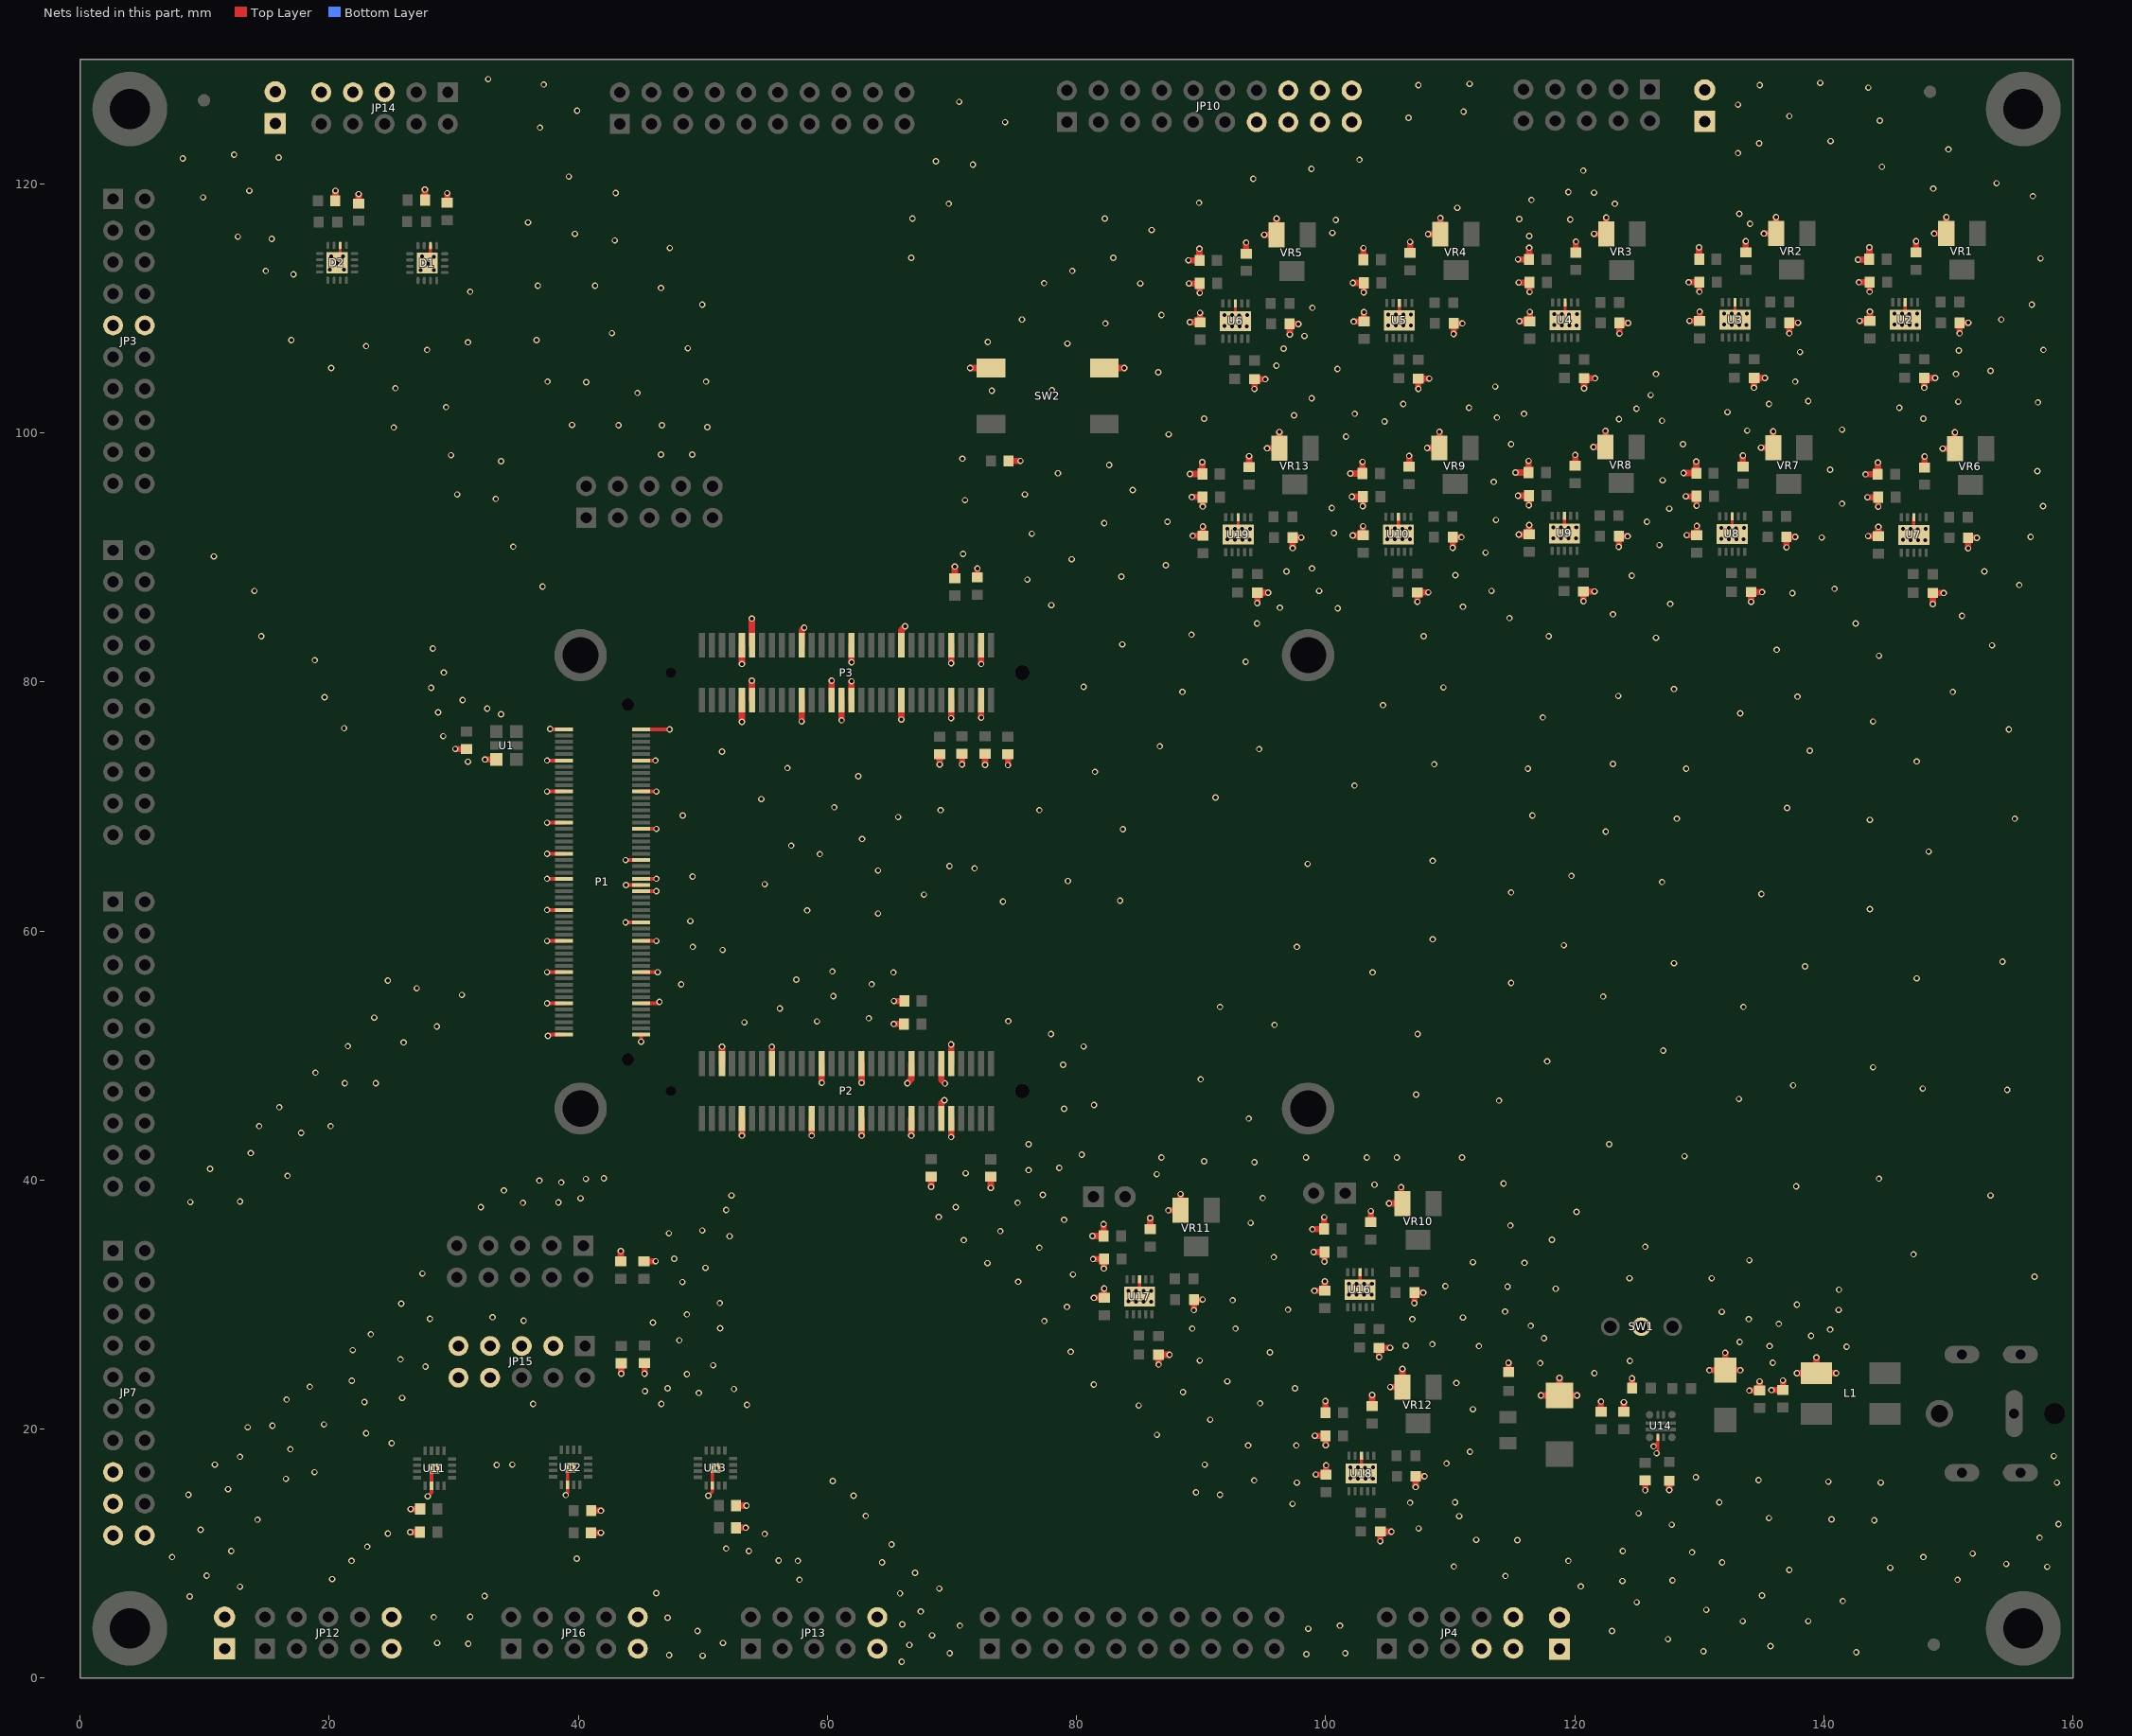
[diagram p0: the nets of this part, all layers, seen from the top]
# Altium PCB MISC82195.PcbDoc (part 4 of 8)
Units mm, origin at the board's own origin, x right, y up, seen from the top; angles counter-clockwise.
Board outline 160 x 130 mm, 4 copper layers (Top Layer, GND, POWER, Bottom Layer); 214 components, 251 nets, 1068 pads, 1218 vias.

## Via types
v1: diameter 0.508, hole 0.305, Top Layer to Bottom Layer, 1218 vias

## Nets (pads, with @x,y where several pads share a name; then routed paths per layer and width w, separated by ;. In a path a pad name is that pad's centre, name@x,y a point inside that pad or via, vN(x,y) a via of type N, cw(c..) or ccw(c..) an arc to the next point about the centre after c; other vN are vias at no path point) (continued)
GND: C1.2 C2.1 C3.1 C4.1 C5.1 C6.1 C7.1 C8.2 C9.1 C10.1 C11.1 C12.2 C13.1 C14.1 C15.1 C16.1 C17.1 C18.1 C19.1 C20.1 C21.1 C22.1 C23.1 C24.1 C25.1 C26.1 C27.1 C28.1 C29.1 C30.1 C31.1 C32.1 C33.1 C34.1 C35.1 C36.1 C37.1 C38.1 C39.1 C40.1 C41.1 C42.1 C43.1 C44.1 C45.1 C46.1 C47.1 C48.1 C49.1 C50.1 C51.1 C52.1 C53.1 C54.1 C55.1 C56.1 C57.1 C58.2 C59.1 C60.2 C61.1 C62.1 C63.1 C64.1 C65.1 C66.1 C67.1 C68.1 C69.1 C70.1 C71.1 C72.1 C73.1 C74.1 C75.1 C76.1 C77.1 C78.1 C79.1 C80.1 C81.1 C82.1 C83.1 D1.14 D1.17 D2.14 D2.17 D3.2 D4.1 JP3.9 JP3.10 JP4.7 JP4.9 JP4.10 JP7.15 JP7.17 JP7.19 JP7.20 JP10.13 JP10.15 JP10.16 JP10.17 JP10.18 JP10.19 JP10.20 JP12.9 JP12.10 JP13.9 JP13.10 JP14.5 JP14.7 JP14.9 JP15.3 JP15.5 JP15.7 JP15.8 JP15.9 JP15.10 JP16.9 JP16.10 JP17.1 JP17.2 JP18.1 JP18.2 JP20.1 JP20.2 JP21.1 JP21.2 L1.3 P1.B1 P1.B2 P1.B11 P1.B12 P1.B21 P1.B22 P1.B32 P1.B33 P1.B42 P1.B43 P1.B49 P1.B50 P1.B51 P1.B53 P1.B60 P1.B63 P1.B69 P1.B70 P1.B79 P1.B80 P1.B89 P1.B90 P1.B99 P1.B100 P2.A5 P2.A10 P2.A15 P2.A24 P2.A25 P2.A33 P2.A34 P2.A43 P2.A44 P2.A49 P2.A50 P2.A51 P2.A52 P3.C9 P3.C10 P3.C11 P3.C12 P3.C21 P3.C22 P3.C28 P3.C30 P3.C31 P3.C32 P3.C41 P3.C42 P3.C51 P3.C52 P3.C57 P3.C58 R7.1 R8.1 R9.1 R10.1 R11.1 R12.1 R19.1 R20.1 R21.1 R22.1 R23.1 R24.1 R31.1 R32.1 R33.1 R34.1 R35.1 R36.1 R39.2 R40.2 R42.1 R49.1 R50.1 R51.1 R52.1 R53.1 R54.1 R57.1 R58.1 SW1.2 SW2.1 SW2.2 U1.3 U2.8 U2.11 U3.8 U3.11 U4.8 U4.11 U5.8 U5.11 U6.8 U6.11 U7.8 U7.11 U8.8 U8.11 U9.8 U9.11 U10.8 U10.11 U11.6 U11.17 U12.6 U12.17 U13.6 U13.17 U14.8 U16.8 U16.11 U17.8 U17.11 U18.8 U18.11 U19.8 U19.11 VR1.3 VR2.3 VR3.3 VR4.3 VR5.3 VR6.3 VR7.3 VR8.3 VR9.3 VR10.3 VR11.3 VR12.3 VR13.3 | length 287.4
  Top Layer w0.254: D2.17@20.891,114.465 D2.14@20.891,115.05 ; D1.17@28.13,114.312 D1.14@28.13,115.024 ; U17.11@85.057,31.387 U17.8@85.057,32.044 ; 92.753,109.771 U6.8@92.753,110.377 ; U19.11@92.982,92.616 U19.8@92.982,93.232 ; U16.11@102.761,31.986 U16.8@102.761,32.603 ; U18.11@102.862,17.188 U18.8@102.862,17.845 ; U10.11@105.834,92.601 U10.8@105.834,93.258 ; U5.11@105.91,109.812 U5.8@105.91,110.428 ; U9.11@119.169,92.667 U9.8@119.169,93.334 ; U4.11@119.22,109.812 U4.8@119.22,110.454 ; v1(126.314,18.618) 126.34,18.618 126.673,18.952 U14.8@126.673,19.339 126.673,18.165 v1(126.568,18.059) ; U8.11@132.631,92.626 U8.8@132.631,93.283 ; U3.11@132.86,109.837 U3.8@132.86,110.479 ; 146.525,109.873 U2.8@146.525,110.479 ; U7.11@147.211,92.565 U7.8@147.211,93.207
  Top Layer w0.279: v1(27.915,14.605) 28.214,14.905 U11.6@28.214,15.443 U11.17@28.214,16.505 ; v1(38.989,14.707) 39.136,14.854 U12.6@39.136,15.519 U12.17@39.136,16.657 ; v1(50.444,14.656) 50.769,14.981 U13.6@50.769,15.468 U13.17@50.769,16.556
  Top Layer w0.305: v1(37.498,54.188) P1.B90@38.866,54.188 ; v1(37.498,56.688) P1.B80@38.866,56.688 ; v1(37.498,59.188) P1.B70@38.866,59.188 ; v1(37.498,61.688) P1.B60@38.866,61.688 ; v1(37.498,64.188) P1.B50@38.866,64.188 ; v1(37.498,66.188) P1.B42@38.866,66.188 ; v1(37.498,68.688) P1.B32@38.866,68.688 ; v1(37.498,71.188) P1.B22@38.866,71.188 ; v1(37.498,73.688) P1.B12@38.866,73.688 ; v1(37.567,51.562) 37.693,51.688 P1.B100@38.866,51.688 ; v1(37.744,76.225) 37.781,76.188 P1.B2@38.866,76.188 ; v1(43.803,60.688) P1.B63@45.038,60.688 ; v1(43.803,65.688) P1.B43@45.038,65.688 ; v1(43.826,63.688) P1.B51@45.038,63.688 ; v1(45.038,51.101) P1.B99@45.038,51.688 ; P1.B89@45.038,54.188 46.391,54.188 v1(46.507,54.305) ; P1.B79@45.038,56.688 v1(46.376,56.688) ; P1.B69@45.038,59.188 v1(46.274,59.188) ; P1.B53@45.038,63.188 v1(46.274,63.188) ; P1.B49@45.038,64.188 v1(46.274,64.188) ; P1.B33@45.038,68.188 v1(46.274,68.188) ; P1.B21@45.038,71.188 v1(46.274,71.188) ; P1.B11@45.038,73.688 v1(46.2,73.688) ; P1.B1@45.038,76.188 v1(47.334,76.188)
  Top Layer w0.508: C59.1@20.503,118.628 v1(20.503,119.436) ; C60.2@22.368,118.414 v1(22.368,119.168) ; v1(26.502,11.72) C50.1@27.282,11.72 ; v1(26.553,13.574) C49.1@27.307,13.574 ; C57.1@27.691,118.679 v1(27.691,119.537) ; C58.2@29.48,118.465 v1(29.48,119.244) ; v1(30.136,74.611) C1.2@31.039,74.611 ; v1(32.515,73.764) U1.3@33.43,73.764 ; C52.1@41.019,11.674 v1(41.819,11.674) ; C51.1@41.044,13.452 v1(41.819,13.452) ; C56.1@43.418,33.481 v1(43.418,34.299) ; v1(43.443,24.444) C61.1@43.443,25.285 ; C55.1@45.272,33.481 v1(46.207,33.481) ; v1(45.323,24.444) C62.1@45.323,25.311 ; P2.A5@51.537,49.338 v1(51.537,50.707) ; C53.1@52.678,12.08 v1(53.452,12.08) ; C54.1@52.678,13.858 v1(53.503,13.858) ; v1(53.137,43.57) P2.A10@53.137,44.938 ; v1(53.137,76.785) P3.C10@53.137,78.539 ; v1(53.137,81.433) P3.C9@53.137,82.939 ; P3.C12@53.937,78.539 v1(53.937,80.099) ; P3.C11@53.937,82.939 v1(53.937,85.078) ; P2.A15@55.537,49.338 v1(55.537,50.707) ; v1(57.937,76.81) P3.C22@57.937,78.539 ; P3.C21@57.937,82.939 57.937,84.15 v1(58.141,84.353) ; v1(58.737,43.57) P2.A24@58.737,44.938 ; v1(59.537,47.803) P2.A25@59.537,49.338 ; P3.C28@60.337,78.539 v1(60.337,80.099) ; v1(61.137,76.912) P3.C30@61.137,78.539 ; P3.C32@61.937,78.539 v1(61.937,80.048) ; v1(61.937,81.573) P3.C31@61.937,82.939 ; v1(62.737,43.57) P2.A34@62.737,44.938 ; v1(62.737,47.803) P2.A33@62.737,49.338 ; v1(65.329,52.527) C6.1@66.153,52.527 ; v1(65.345,54.372) C4.1@66.168,54.372 ; v1(65.937,76.963) P3.C42@65.937,78.539 ; P3.C41@65.937,82.939 65.937,84.149 v1(66.243,84.455) ; v1(66.421,47.777) 66.737,48.094 P2.A43@66.737,49.338 ; v1(66.737,43.57) P2.A44@66.737,44.938 ; v1(68.326,39.446) C5.1@68.326,40.27 ; v1(69.012,73.355) C12.2@69.012,74.205 ; P2.A50@69.137,44.938 69.137,46.15 v1(69.393,46.406) ; P2.A49@69.137,49.338 69.137,48.058 v1(69.444,47.752) ; v1(69.937,43.448) P2.A52@69.937,44.938 ; P2.A51@69.937,49.338 v1(69.937,50.887) ; v1(69.937,77.078) P3.C52@69.937,78.539 ; v1(69.937,81.497) P3.C51@69.937,82.939 ; C11.1@70.231,88.33 v1(70.231,89.256) ; v1(70.806,73.371) C9.1@70.806,74.215 ; v1(71.461,105.196) SW2.1@73.123,105.196 ; C10.1@72.034,88.381 v1(72.034,89.103) ; v1(72.337,77.116) P3.C58@72.337,78.539 ; v1(72.337,81.434) P3.C57@72.337,82.939 ; v1(72.66,73.339) C2.1@72.66,74.215 ; v1(73.117,39.361) C7.1@73.117,40.255 ; v1(74.489,73.314) C3.1@74.489,74.189 ; C8.2@74.538,97.739 v1(75.489,97.739) ; v1(81.28,35.509) C72.1@82.274,35.509 ; v1(81.331,33.655) C73.1@82.198,33.655 v1(82.198,32.896) ; v1(81.393,30.545) C71.1@82.22,30.545 v1(82.22,31.293) ; C72.1@82.172,35.509 v1(82.172,36.452) ; SW2.2@82.223,105.196 v1(83.835,105.196) ; C78.1@85.92,36.057 v1(85.92,36.939) ; v1(86.581,25.179) R53.1@86.581,25.967 v1(87.461,25.967) ; v1(87.374,37.569) VR11.3@88.353,37.569 v1(88.353,38.874) ; v1(88.976,113.843) C29.1@89.869,113.843 v1(89.869,114.786) ; v1(89.027,111.989) C30.1@89.894,111.989 v1(89.894,111.23) ; v1(89.089,108.879) C28.1@89.916,108.879 v1(89.916,109.626) ; v1(89.103,96.698) C81.1@90.097,96.698 v1(90.097,97.641) ; v1(89.256,94.844) C82.1@90.123,94.844 v1(90.123,94.085) ; v1(89.318,91.734) C80.1@90.145,91.734 v1(90.145,92.481) ; v1(89.417,29.549) R50.1@89.417,30.404 v1(90.119,30.404) ; C35.1@93.617,114.39 v1(93.617,115.273) ; C83.1@93.845,97.245 v1(93.845,98.128) ; v1(94.277,103.513) R23.1@94.277,104.301 v1(95.157,104.301) ; v1(94.506,86.327) R58.1@94.506,87.156 v1(95.386,87.156) ; v1(95.07,115.902) VR5.3@96.05,115.902 v1(96.05,117.208) ; v1(95.299,98.757) VR13.3@96.278,98.757 v1(96.278,100.063) ; v1(97.113,107.883) R20.1@97.113,108.737 v1(97.815,108.737) ; v1(97.342,90.738) R57.1@97.342,91.592 v1(98.044,91.592) ; v1(98.933,36.043) C69.1@99.927,36.043 ; v1(99.035,34.214) C70.1@99.902,34.214 v1(99.902,33.455) ; v1(99.097,31.104) C68.1@99.924,31.104 v1(99.924,31.852) ; v1(99.136,19.456) C76.1@100.003,19.456 v1(100.003,18.698) ; v1(99.198,16.346) C74.1@100.025,16.346 v1(100.025,17.094) ; C69.1@99.876,36.068 v1(99.876,37.011) ; C75.1@99.978,21.311 v1(99.978,22.254) ; v1(101.981,96.723) C44.1@102.975,96.723 ; v1(102.108,94.869) C45.1@102.975,94.869 v1(102.975,94.11) ; v1(102.17,91.759) C43.1@102.997,91.759 v1(102.997,92.507) ; v1(102.184,112.039) C27.1@103.051,112.039 v1(103.051,111.281) ; v1(102.246,108.929) C25.1@103.073,108.929 v1(103.073,109.677) ; C44.1@102.95,96.723 v1(102.95,97.666) ; C26.1@103.026,113.894 v1(103.026,114.837) ; C77.1@103.624,36.616 v1(103.624,37.498) ; C79.1@103.726,21.858 v1(103.726,22.741) ; v1(104.285,25.773) R52.1@104.285,26.526 v1(105.165,26.526) ; v1(104.386,10.99) R54.1@104.386,11.769 v1(105.266,11.769) ; v1(105.078,38.128) 106.057,38.128 v1(106.057,39.433) ; v1(105.179,23.37) VR12.3@106.159,23.37 ; VR12.3@106.159,23.523 v1(106.159,24.828) ; C48.1@106.698,97.271 v1(106.698,98.153) ; C34.1@106.774,114.441 v1(106.774,115.324) ; v1(107.121,30.108) R49.1@107.121,30.963 v1(107.823,30.963) ; v1(107.222,15.351) R51.1@107.222,16.205 v1(107.925,16.205) ; v1(107.358,86.419) R36.1@107.358,87.181 v1(108.238,87.181) ; v1(107.434,103.523) R22.1@107.434,104.352 v1(108.314,104.352) ; v1(108.151,98.783) VR9.3@109.131,98.783 v1(109.131,100.088) ; v1(108.227,115.953) VR4.3@109.207,115.953 v1(109.207,117.259) ; v1(110.194,90.763) R33.1@110.194,91.618 v1(110.896,91.618) ; v1(110.27,107.934) R19.1@110.27,108.788 v1(110.973,108.788) ; R42.1@114.681,24.579 v1(114.681,25.324) ; v1(115.24,96.799) C41.1@116.234,96.799 ; v1(115.443,94.945) C42.1@116.31,94.945 v1(116.31,94.187) ; v1(115.443,113.919) C20.1@116.437,113.919 ; v1(115.494,112.065) C21.1@116.361,112.065 v1(116.361,111.306) ; v1(115.505,91.835) C40.1@116.332,91.835 v1(116.332,92.583) ; v1(115.556,108.955) C19.1@116.383,108.955 v1(116.383,109.703) ; C41.1@116.285,96.799 v1(116.285,97.743) ; C20.1@116.335,113.919 v1(116.335,114.862) ; v1(117.273,22.706) D3.2@118.77,22.706 ; v1(118.77,24.105) D3.2@118.77,22.706 ; C47.1@120.033,97.347 v1(120.033,98.23) ; C24.1@120.083,114.467 v1(120.083,115.349) ; v1(120.191,22.706) D3.2@118.77,22.706 ; v1(120.693,86.469) R35.1@120.693,87.258 v1(121.573,87.258) ; v1(120.744,103.564) R12.1@120.744,104.377 v1(121.624,104.377) ; v1(121.486,98.859) VR8.3@122.466,98.859 v1(122.466,100.164) ; v1(121.537,115.979) VR3.3@122.516,115.979 v1(122.516,117.284) ; C64.1@122.098,21.401 v1(122.098,22.225) ; v1(123.529,90.839) R32.1@123.529,91.694 v1(124.231,91.694) ; v1(123.58,107.959) R9.1@123.58,108.814 v1(124.282,108.814) ; C63.1@123.936,21.391 v1(123.936,22.158) ; R39.2@124.596,23.292 v1(124.596,24.071) ; v1(125.654,15.088) C67.1@125.654,15.886 ; v1(127.584,15.113) R40.2@127.584,15.858 ; v1(128.727,96.774) C38.1@129.721,96.774 ; v1(128.905,94.894) C39.1@129.772,94.894 v1(129.772,94.136) ; v1(128.967,91.784) C37.1@129.794,91.784 v1(129.794,92.532) ; v1(129.134,112.09) C18.1@130.001,112.09 v1(130.001,111.332) ; v1(129.196,108.98) C16.1@130.023,108.98 v1(130.023,109.728) ; C38.1@129.747,96.749 v1(129.747,97.692) ; C17.1@129.975,113.944 v1(129.975,114.888) ; v1(130.791,24.733) D4.1@132.08,24.733 ; v1(132.08,26.137) D4.1@132.08,24.733 ; v1(133.293,24.733) D4.1@132.08,24.733 ; C46.1@133.495,97.296 v1(133.495,98.179) ; C23.1@133.723,114.492 v1(133.723,115.375) ; v1(134.006,23.093) C66.1@134.832,23.093 v1(134.832,23.834) ; v1(134.155,86.419) R34.1@134.155,87.207 v1(135.035,87.207) ; v1(134.384,103.614) R11.1@134.384,104.403 v1(135.264,104.403) ; v1(134.948,98.808) VR7.3@135.928,98.808 v1(135.928,100.114) ; v1(135.177,116.004) VR2.3@136.156,116.004 v1(136.156,117.309) ; v1(135.777,23.128) C65.1@136.703,23.128 v1(136.703,23.901) ; v1(136.991,90.789) R31.1@136.991,91.643 v1(137.693,91.643) ; v1(137.22,107.984) R8.1@137.22,108.839 v1(137.922,108.839) ; v1(137.82,24.485) L1.3@139.388,24.485 ; v1(139.388,25.749) L1.3@139.388,24.485 ; v1(140.969,24.485) L1.3@139.388,24.485 ; v1(142.723,113.894) C14.1@143.717,113.894 ; v1(142.799,112.09) C15.1@143.666,112.09 v1(143.666,111.332) ; v1(142.861,108.98) C13.1@143.688,108.98 v1(143.688,109.728) ; v1(143.332,96.672) C32.1@144.326,96.672 v1(144.326,97.616) ; v1(143.485,94.818) C33.1@144.352,94.818 v1(144.352,94.06) ; v1(143.547,91.708) C31.1@144.374,91.708 v1(144.374,92.456) ; C14.1@143.64,113.944 v1(143.64,114.888) ; C22.1@147.388,114.492 v1(147.388,115.375) ; v1(148.049,103.614) R10.1@148.049,104.403 v1(148.929,104.403) ; C36.1@148.074,97.22 v1(148.074,98.103) ; v1(148.735,86.241) R24.1@148.735,87.131 v1(149.615,87.131) ; v1(148.842,116.004) VR1.3@149.821,116.004 v1(149.821,117.309) ; v1(149.528,98.732) VR6.3@150.507,98.732 v1(150.507,100.037) ; v1(150.885,107.984) R7.1@150.885,108.839 v1(151.587,108.839) ; v1(151.571,90.712) R21.1@151.571,91.567 v1(152.273,91.567)
  Bottom Layer w0.305: v1@37.719,76.2 v1(37.744,76.225)
  other v1: 65.964,1.321 49.987,1.803 47.295,1.854 98.45,1.93 69.825,2.007 101.575,2.007 142.596,2.083 130.327,2.159 135.712,2.565 66.573,2.667 31.166,2.769 28.677,2.819 51.613,2.819 127.483,3.124 68.402,3.429 49.581,3.785 122.987,3.785 98.603,3.962 70.637,4.216 101.143,4.216 66.015,4.318 133.477,4.572 138.735,4.572 47.168,4.851 28.397,4.902 31.318,4.928 67.488,5.359 130.556,5.486 124.968,6.096 141.503,6.198 8.814,6.553 32.487,6.604 135.026,6.629 65.837,6.807 46.253,6.833 68.986,7.188 12.852,7.341 120.472,7.366 123.825,7.798 127.838,7.849 57.76,7.899 150.724,7.899 20.244,7.95 114.427,8.204 10.16,8.23 67.031,8.458 137.211,8.687 145.313,8.865 157.912,8.941 110.287,8.966 154.635,9.169 64.389,9.296 131.826,9.296 21.793,9.423 57.633,9.423 119.482,9.423 56.083,9.449 39.878,9.601 7.391,9.728 147.98,9.728 151.943,10.008 129.413,10.109 12.141,10.211 53.696,10.211 123.85,10.211 51.867,10.414 23.063,10.566 65.151,10.744 115.392,11.074 112.09,11.1 157.302,11.278 54.966,11.582 24.714,11.608 9.677,11.913 107.467,12.014 127.787,12.319 158.826,12.37 144.043,12.675 14.249,12.725 140.614,12.751 135.585,12.852 110.719,13.005 63.068,13.03 125.12,13.233 97.333,13.995 106.782,14.097 110.388,14.122 131.597,14.122 62.103,14.656 8.712,14.732 91.516,14.732 89.586,14.91 11.887,15.164 97.688,15.697 144.551,15.697 158.699,15.697 140.36,15.773 60.427,15.824 94.259,15.875 134.747,15.9 16.535,16.002 102.591,16.027 103.2,16.027 103.784,16.027 101.981,16.053 129.718,16.129 18.821,16.535 28.473,16.84 51.029,16.84 103.175,16.891 39.395,16.916 101.981,16.916 102.591,16.916 103.81,16.916 33.452,17.12 10.82,17.145 34.696,17.145 90.297,17.145 109.703,17.247 12.852,17.78 158.445,17.831 111.582,18.186 16.891,18.39 93.777,18.694 97.638,18.694 25.019,18.872 86.462,19.533 22.962,19.66 13.462,20.142 15.443,20.269 19.583,20.371 90.729,20.752 111.811,21.59 84.988,21.895 53.543,21.946 36.373,22.022 46.66,22.022 94.742,22.073 22.835,22.174 16.586,22.377 25.857,22.504 49.682,22.911 88.544,22.962 45.364,23.038 52.502,23.216 47.168,23.266 97.536,23.266 18.44,23.393 81.382,23.571 110.49,23.698 92.1,23.825 21.819,23.876 48.717,24.409 121.564,24.486 27.737,25.019 50.825,25.121 117.221,25.298 135.89,25.324 124.409,25.476 89.891,25.502 25.73,25.603 95.529,26.162 79.527,26.213 21.895,26.34 141.808,26.619 112.293,26.67 135.636,26.67 106.426,26.695 108.56,26.822 133.223,27 48.108,27.127 117.526,27.305 138.963,27.483 23.343,27.61 140.487,27.991 89.281,28.067 92.761,28.067 51.384,28.092 116.459,28.296 136.373,28.448 45.999,28.55 77.419,28.677 35.611,28.702 106.959,28.829 133.96,28.829 28.092,28.854 111.023,28.956 33.122,28.981 48.717,29.21 131.801,29.413 114.402,29.439 141.173,29.566 96.977,29.591 79.223,29.82 137.82,29.997 25.781,30.074 51.359,30.124 84.785,30.226 85.395,30.226 85.979,30.226 84.176,30.251 92.532,30.353 102.489,30.785 103.099,30.785 103.683,30.785 101.879,30.81 85.369,31.09 84.176,31.115 84.785,31.115 86.004,31.115 141.199,31.191 118.466,31.267 114.605,31.445 109.601,31.471 103.073,31.648 101.879,31.674 102.489,31.674 103.708,31.674 48.362,31.801 75.311,31.826 124.384,32.106 130.988,32.106 156.896,32.233 79.705,32.41 27.483,32.487 50.216,32.944 72.847,33.325 115.951,33.35 111.811,33.401 134.01,33.553 47.701,33.68 95.834,33.807 147.193,34.036 77.013,34.569 125.654,34.646 70.942,35.179 118.161,35.204 52.146,35.484 47.269,35.712 73.889,35.89 49.962,35.941 114.833,36.347 93.98,36.551 78.994,36.805 68.936,37.033 120.142,37.44 51.867,37.592 32.182,37.821 70.307,37.821 35.56,38.176 75.26,38.176 38.405,38.202 8.865,38.227 12.852,38.278 40.183,38.532 94.945,38.557 52.299,38.76 153.365,38.76 77.292,38.811 34.036,39.167 137.77,39.497 103.911,39.624 114.275,39.726 38.633,39.802 36.881,39.954 40.615,40.081 144.424,40.107 42.062,40.132 16.662,40.335 86.436,40.462 71.095,40.538 76.149,40.792 10.439,40.894 78.613,40.97 94.285,41.427 90.246,41.504 86.817,41.808 98.425,41.808 103.302,41.808 105.715,41.808 110.947,41.808 128.803,41.91 80.416,42.037 13.716,42.164 76.149,42.875 122.758,42.875 17.755,43.79 14.376,44.323 20.117,44.323 93.828,44.933 78.994,45.72 16.002,45.847 81.407,46.025 113.919,46.38 133.172,46.507 107.264,46.863 154.711,47.244 147.93,47.346 137.516,47.6 21.26,47.777 23.749,47.777 89.967,48.082 18.898,48.616 143.942,49.047 78.918,49.251 117.78,49.53 127.102,50.394 80.569,50.724 21.514,50.749 25.984,51.054 77.953,51.714 107.391,51.714 28.651,52.324 95.885,52.451 53.34,52.654 59.157,52.73 74.524,52.756 63.322,52.984 23.622,53.035 56.185,53.772 91.516,53.899 133.528,53.899 122.276,54.737 60.477,54.762 30.658,54.864 27.026,55.397 48.26,55.702 63.551,55.728 114.884,55.829 24.714,56.007 57.506,56.083 147.447,56.185 65.303,56.667 103.759,56.667 60.401,56.744 138.481,57.15 127.965,57.404 154.33,57.531 51.587,58.471 49.2,58.725 97.688,58.725 119.126,58.852 108.585,59.334 48.997,60.782 64.059,61.392 58.369,61.646 143.688,61.747 74.092,62.357 83.49,62.433 67.742,62.916 134.976,62.967 114.884,63.094 54.966,63.754 127,63.932 79.299,64.008 49.174,64.364 119.736,64.414 64.059,64.846 71.806,65.024 69.799,65.202 98.552,65.38 108.585,65.634 59.385,66.167 148.412,66.37 57.099,66.853 62.789,67.386 122.479,67.97 83.718,68.174 143.688,68.91 128.194,69.012 155.321,69.012 65.684,69.139 48.387,69.266 116.586,69.266 69.088,69.698 77.013,69.698 137.033,69.875 60.554,69.926 54.686,70.587 91.161,70.714 102.311,71.679 62.484,72.415 81.483,72.771 116.23,73.025 128.93,73.025 56.794,73.076 108.712,73.381 123.063,73.406 31.14,73.584 147.447,73.609 51.537,74.397 138.862,74.473 94.666,74.6 86.69,74.828 29.159,75.641 154.838,76.175 21.209,76.276 143.942,76.81 117.424,77.14 33.807,77.394 133.274,77.47 28.753,77.546 32.69,77.851 104.597,78.13 30.709,78.537 19.634,78.765 137.871,78.816 123.495,78.867 88.494,79.197 150.343,79.197 127.965,79.426 28.194,79.527 109.449,79.553 80.569,79.604 29.21,80.747 93.574,81.61 18.847,81.737 144.424,82.093 136.195,82.575 28.321,82.677 153.492,82.931 83.668,83.007 126.517,83.541 14.554,83.668 107.874,83.668 117.907,83.668 89.23,83.795 94.488,84.684 142.545,84.684 114.757,85.115 151.079,85.293 123.063,85.42 100.965,85.903 96.317,85.954 111.023,86.03 77.978,86.157 127.66,86.258 137.465,87.122 13.995,87.3 99.466,87.3 113.309,87.3 140.843,87.478 37.135,87.655 155.677,87.782 76.048,88.214 83.591,88.443 124.562,88.519 110.414,88.57 96.85,88.875 152.883,88.875 98.908,89.103 87.173,89.357 79.604,89.84 10.744,90.068 70.891,90.272 112.827,90.373 34.773,90.856 126.797,90.983 146.939,91.389 147.549,91.389 148.133,91.389 92.71,91.415 93.32,91.415 93.904,91.415 146.329,91.415 92.1,91.44 105.562,91.44 106.172,91.44 106.756,91.44 104.953,91.465 132.359,91.465 132.969,91.465 133.553,91.465 131.75,91.491 118.897,91.516 119.507,91.516 120.091,91.516 118.288,91.542 139.827,91.592 156.591,91.643 76.403,91.897 100.66,91.948 147.523,92.253 93.294,92.278 146.329,92.278 146.939,92.278 148.158,92.278 92.1,92.304 92.71,92.304 93.929,92.304 106.147,92.304 104.953,92.329 105.562,92.329 106.782,92.329 132.944,92.329 131.75,92.354 132.359,92.354 133.579,92.354 119.482,92.38 118.288,92.405 118.897,92.405 120.117,92.405 82.22,92.735 87.3,92.862 125.781,92.862 113.665,92.989 127.584,93.904 100.482,93.955 157.582,94.107 141.453,94.31 71.044,94.59 33.376,94.691 30.277,95.047 75.844,95.047 84.506,95.402 113.487,96.063 127.051,96.19 78.511,96.749 157.124,96.926 140.487,97.028 82.626,97.409 33.807,97.714 70.841,97.917 29.794,98.196 46.634,98.247 49.149,98.247 114.884,99.085 128.676,99.085 101.625,99.695 87.401,99.873 133.833,100.178 141.453,100.254 25.197,100.432 50.368,100.457 43.231,100.609 46.711,100.609 39.497,100.635 104.724,100.914 127,100.965 123.546,101.092 90.246,101.143 147.98,101.143 113.741,101.219 97.46,101.397 102.337,101.524 115.926,101.524 132.258,101.651 124.943,101.93 111.506,102.006 146.05,102.006 29.388,102.057 106.223,102.311 135.585,102.311 157.175,102.438 150.774,102.489 138.735,102.54 98.882,102.768 126.086,103.022 44.755,103.2 73.203,103.378 78.029,103.429 25.324,103.581 113.614,103.708 40.64,104.064 37.541,104.115 50.267,104.115 137.693,104.115 126.517,104.724 150.597,104.724 86.563,104.851 153.365,104.978 100.94,105.131 20.168,105.207 96.037,105.385 138.074,106.477 150.825,106.604 27.864,106.655 157.607,106.655 96.622,106.756 48.793,106.782 22.962,106.959 79.273,107.163 31.14,107.264 72.873,107.29 16.967,107.442 36.652,107.442 98.298,107.772 42.697,108.001 92.481,108.56 93.091,108.56 93.675,108.56 91.872,108.585 105.639,108.61 106.248,108.61 106.832,108.61 105.029,108.636 118.948,108.636 119.558,108.636 120.142,108.636 118.339,108.661 132.588,108.661 133.198,108.661 133.782,108.661 146.253,108.661 146.863,108.661 147.447,108.661 131.978,108.687 145.644,108.687 82.321,108.788 75.616,109.093 154.229,109.093 93.066,109.423 86.817,109.449 91.872,109.449 92.481,109.449 93.701,109.449 106.223,109.474 105.029,109.499 105.639,109.499 106.858,109.499 119.532,109.499 118.339,109.525 118.948,109.525 120.167,109.525 133.172,109.525 146.837,109.525 131.978,109.55 132.588,109.55 133.807,109.55 145.644,109.55 146.253,109.55 147.472,109.55 98.933,110.033 49.962,110.287 156.693,110.287 31.318,111.328 46.634,111.633 36.754,111.811 41.351,111.811 85.115,111.989 77.394,112.014 17.145,112.725 14.91,113.005 79.654,113.005 27.356,113.081 28.397,113.081 20.066,113.106 21.184,113.106 27.915,113.589 20.625,113.614 157.378,113.995 66.726,114.046 82.956,114.046 28.397,114.122 21.107,114.148 27.457,114.148 20.168,114.173 47.346,114.833 42.926,115.443 15.392,115.57 12.675,115.748 116.332,115.799 39.726,115.976 100.533,116.053 86.03,116.281 134.061,116.789 35.966,116.891 100.813,117.094 119.634,117.119 115.545,117.17 66.827,117.196 82.271,117.196 133.198,117.577 110.566,118.059 69.748,118.389 123.215,118.389 89.84,118.466 116.51,118.694 9.881,118.897 156.769,118.999 43.002,119.253 121.539,119.278 119.482,119.329 13.589,119.431 148.768,119.609 153.848,120.04 94.183,120.396 39.243,120.574 120.675,121.056 98.857,121.183 144.653,121.361 71.679,121.539 68.707,121.793 102.718,121.92 8.255,122.022 15.951,122.098 12.37,122.326 133.096,122.453 149.987,122.758 134.798,123.241 140.538,123.419 36.932,124.511 74.27,124.943 144.475,125.07 106.655,125.298 137.211,125.425 111.074,125.781 39.903,125.857 133.096,126.34 70.587,126.568 143.561,127.711 107.442,127.914 134.849,127.914 37.236,127.965 111.557,128.016 139.7,128.092 32.766,128.397